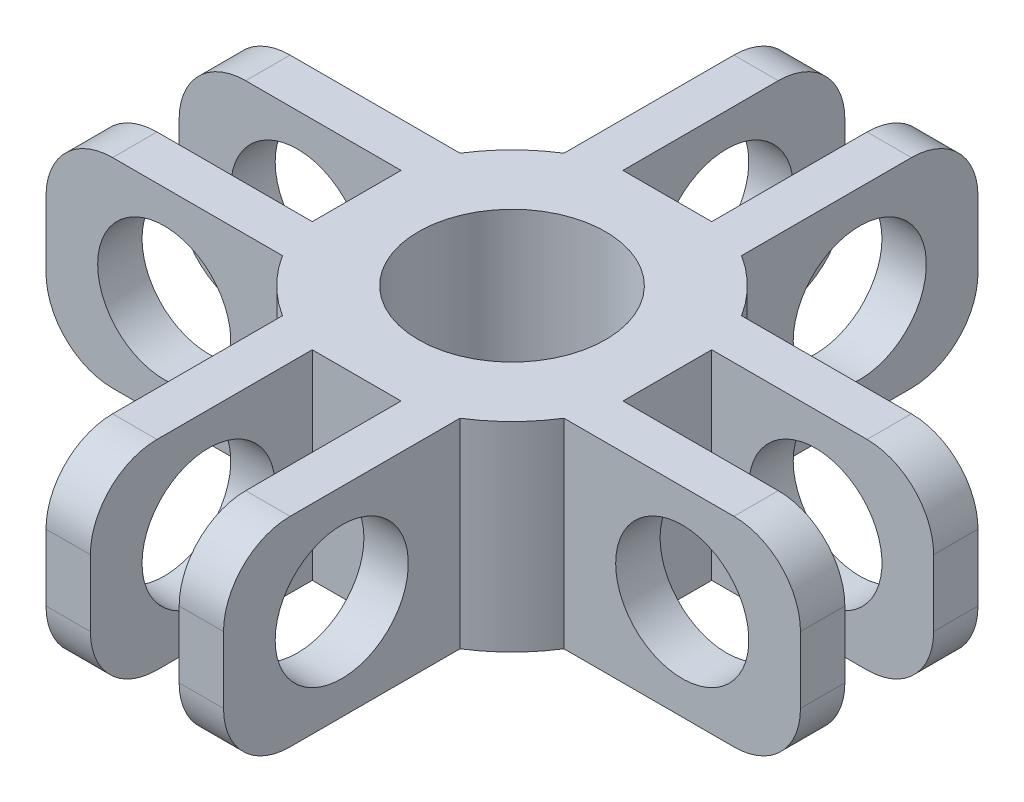
from build123d import *

# Parameters (mm, degrees)
BOSS_EXTRUDE1_DEPTH     = 11.43
SKETCH2_R               = 9.525
BOSS_EXTRUDE2_DEPTH     = 11.43
SKETCH8_R               = 3.81
CUT_EXTRUDE6_DEPTH      = 37.167138399
SKETCH9_R               = 3.81
CUT_EXTRUDE7_DEPTH      = 37.167138399
F_1_2_13_TAPPED_HOLE1_D = 10.71626
SKETCH12_W              = 25.4
SKETCH12_H              = 5.08
CUT_EXTRUDE8_DEPTH      = 33.602164039
CIRPATTERN1_COUNT       = 4
FILLET1_R               = 3.81
SCALE1_SCALE            = 2


with BuildPart() as part:
    # Sketch1 → Boss-Extrude1 (new body)
    with BuildSketch(Plane(origin=(0, 0, 0), x_dir=(1, 0, 0), z_dir=(0, 1, 0))):
        Polygon((-5.08, 21.59), (5.08, 21.59), (5.08, 5.08), (21.59, 5.08), (21.59, -5.08), (5.08, -5.08), (5.08, -21.59), (-5.08, -21.59), (-5.08, -5.08), (-21.59, -5.08), (-21.59, 5.08), (-5.08, 5.08), align=None)
    extrude(amount=BOSS_EXTRUDE1_DEPTH)

    # Sketch2 → Boss-Extrude2 (add)
    with BuildSketch(Plane(origin=(0, 11.43, 0), x_dir=(1, 0, 0), z_dir=(0, 1, 0))):
        Circle(SKETCH2_R)
    extrude(amount=-BOSS_EXTRUDE2_DEPTH)

    # Sketch8 → Cut-Extrude6 (cut, through all)
    with BuildSketch(Plane.ZY.offset(5.08)):
        with Locations((14.823623369, 5.715)):
            Circle(SKETCH8_R)
        with Locations((-14.823623369, 5.715)):
            Circle(SKETCH8_R)
    extrude(amount=-CUT_EXTRUDE6_DEPTH, mode=Mode.SUBTRACT)

    # Sketch9 → Cut-Extrude7 (cut, through all)
    with BuildSketch(Plane(origin=(0, 0, -5.08), x_dir=(-1, 0, 0), z_dir=(0, 0, -1))):
        with Locations((14.823623369, 5.715)):
            Circle(SKETCH9_R)
        with Locations((-14.823623369, 5.715)):
            Circle(SKETCH9_R)
    extrude(amount=-CUT_EXTRUDE7_DEPTH, mode=Mode.SUBTRACT)

    # 1/2-13 Tapped Hole1 (through all)
    with Locations(Plane(origin=(0, 11.43, 0), x_dir=(1, 0, 0), z_dir=(0, 1, 0))):
        with Locations((0, 0)):
            Hole(F_1_2_13_TAPPED_HOLE1_D / 2)

    # Sketch12 → Cut-Extrude8 (cut, through all)
    with BuildSketch(Plane(origin=(0, 11.43, 0), x_dir=(1, 0, 0), z_dir=(0, 1, 0))):
        with Locations((-21.59, 0)):
            Rectangle(SKETCH12_W, SKETCH12_H)
    cut_extrude8 = extrude(amount=-CUT_EXTRUDE8_DEPTH, mode=Mode.SUBTRACT)

    # CirPattern1: Cut-Extrude8 ×4 about axis
    cirpattern1_axis = Axis((0, 0, 0), (0, 1, 0))
    for i in range(1, CIRPATTERN1_COUNT):
        add(cut_extrude8.rotate(cirpattern1_axis, i * 360 / CIRPATTERN1_COUNT), mode=Mode.SUBTRACT)

    # Fillet1
    fillet1_edges = [part.edges().sort_by_distance(p)[0] for p in [
        (-21.59, 0, 3.81),
        (-21.59, 11.43, 3.81),
        (21.59, 0, 3.81),
        (-3.81, 0, 21.59),
        (3.81, 0, 21.59),
        (3.81, 11.43, 21.59),
        (-21.59, 0, -3.81),
        (21.59, 0, -3.81),
        (21.59, 11.43, -3.81),
        (3.81, 0, -21.59),
        (-21.59, 11.43, -3.81),
        (-3.81, 0, -21.59),
        (-3.81, 11.43, -21.59),
        (-3.81, 11.43, 21.59),
        (21.59, 11.43, 3.81),
        (3.81, 11.43, -21.59),
    ]]
    fillet(fillet1_edges, radius=FILLET1_R)


with BuildPart() as part_1:
    # Scale1: scaled about (0, 0, 0)
    add(part.part.scale(SCALE1_SCALE))


solid = part_1.part
